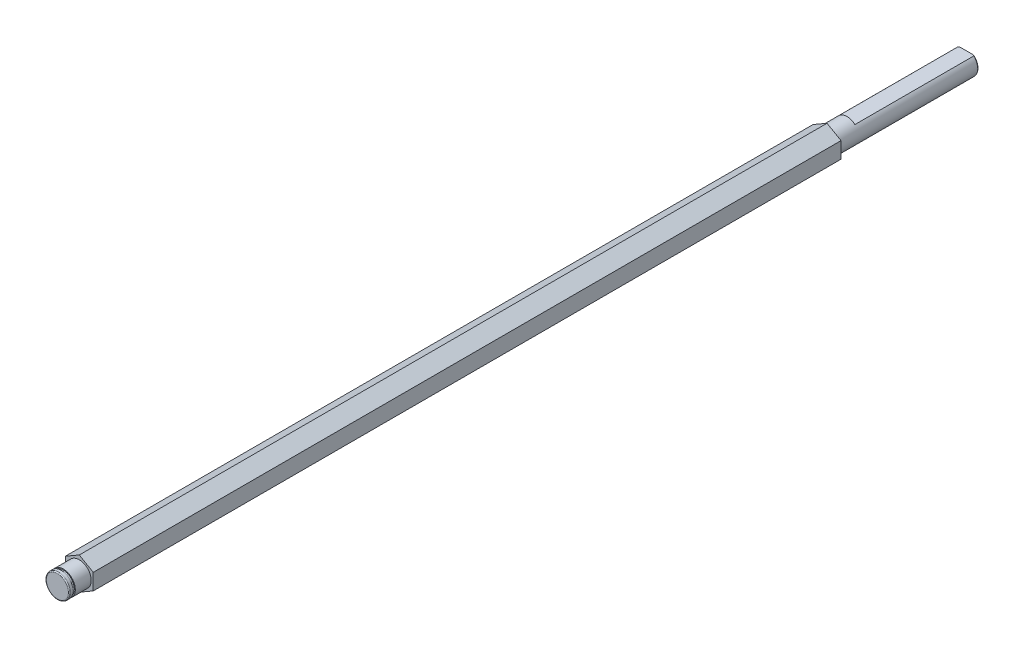
SolidWorks part; units mm, degrees
ref_plane "前视基准面" through (0, 0, 0) normal (0, 0, 1) x (1, 0, 0)
ref_plane "上视基准面" through (0, 0, 0) normal (0, 1, 0) x (1, 0, 0)
ref_plane "右视基准面" through (0, 0, 0) normal (1, 0, 0) x (0, 0, -1)
sketch "草图1" plane through (0, 0, 0) normal (0, 0, 1) x (1, 0, 0)
  line L1 (7, -4.0415) -> (7, 4.0415)
  line L2 (7, 4.0415) -> (0, 8.0829)
  line L3 (0, 8.0829) -> (-7, 4.0415)
  line L4 (-7, 4.0415) -> (-7, -4.0415)
  line L5 (-7, -4.0415) -> (0, -8.0829)
  line L6 (0, -8.0829) -> (7, -4.0415)
  circle A0 centre (0, 0) radius 7 construction
  dimension "D1" = 14
extrude "凸台-拉伸1" add sketch "草图1" along normal blind 375
sketch "草图2" plane through (0, 0, 0) normal (0, 0, -1) x (-1, 0, 0)
  circle A0 centre (0, 0) radius 6
  dimension "D1" = 12
extrude "凸台-拉伸2" add sketch "草图2" along normal blind 70
sketch "草图3" plane through (0, 0, 375) normal (0, 0, 1) x (1, 0, 0)
  circle A0 centre (0, 0) radius 6
  dimension "D1" = 12
extrude "凸台-拉伸3" add sketch "草图3" along normal blind 11
fillet "圆角1" radius 0.5 1 edges at (-6, 0, -70)
sketch "草图6" plane through (0, 0, 0) normal (0, 1, 0) x (1, 0, 0)
  line L0 (0, -418.9281) -> (0, -404.8793) construction
  line L1 (6, -386) -> (6, -375) construction
  line L2 (5.5, -383) -> (6.5, -383)
  line L3 (5.5, -383) -> (5.5, -384.1)
  line L4 (5.5, -384.1) -> (6.5, -384.1)
  line L5 (6.5, -383) -> (6.5, -384.1)
  line L6 (5.5, -383) -> (6.5, -384.1) construction
  line L7 (5.5, -384.1) -> (6.5, -383) construction
  line L8 (-6, -386) -> (6, -386) construction
  point P3 (6, -383.55)
  dimension "D1" = 3
  dimension "D2" = 1
  dimension "D3" = 1.1
revolve "切除-旋转2" cut sketch "草图6" angle 360 about L0
fillet "圆角2" radius 0.5 1 edges at (6, 0, 386)
sketch "草图7" plane through (0, 0, -70) normal (0, 0, -1) x (-1, 0, 0)
  line L1 (5, 6.5) -> (-5, 6.5)
  line L2 (5, 6.5) -> (5, 4.5)
  line L3 (5, 4.5) -> (-5, 4.5)
  line L4 (-5, 6.5) -> (-5, 4.5)
  line L5 (5, 6.5) -> (-5, 4.5) construction
  line L6 (5, 4.5) -> (-5, 6.5) construction
  circle A0 centre (0, 0) radius 5.5 construction
  point P0 (0, 5.5)
  dimension "D1" = 10
  dimension "D2" = 2
extrude "切除-拉伸1" cut sketch "草图7" against normal blind 60
